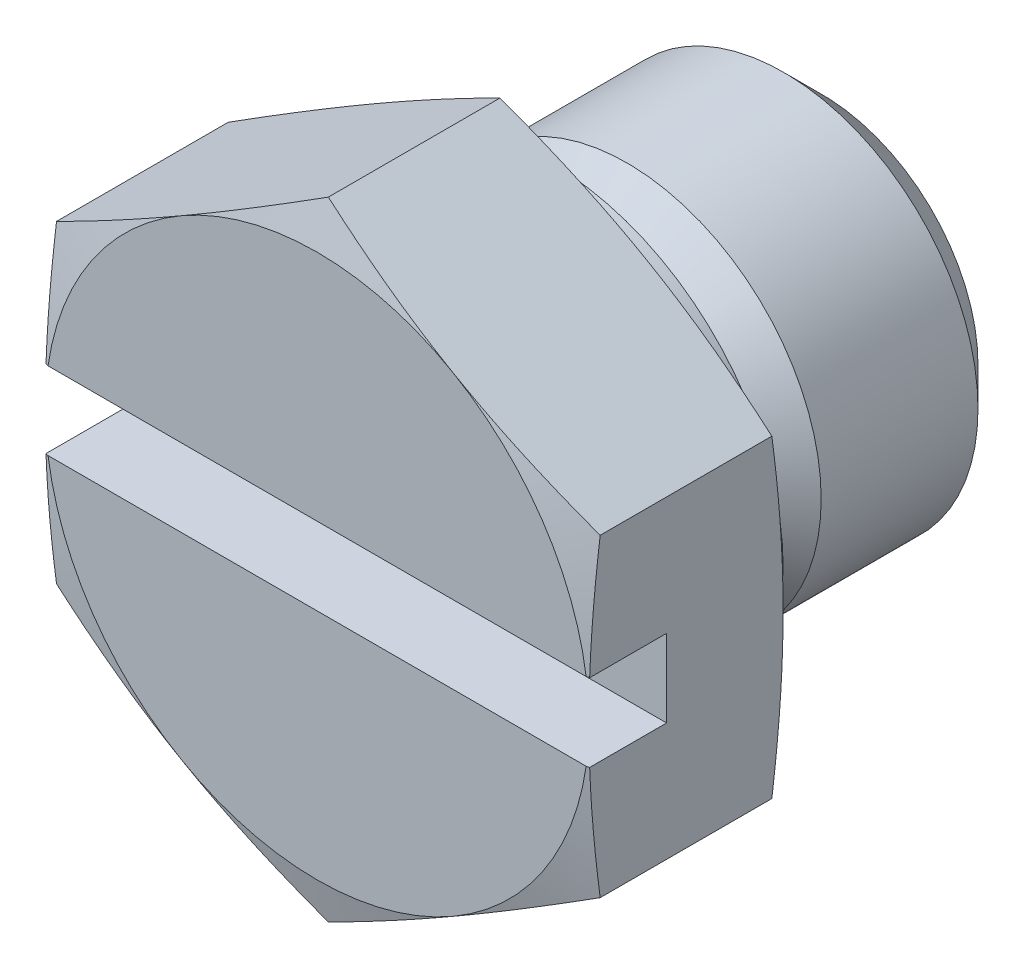
from build123d import *

# Parameters (mm, degrees)
SKETCH_2_R          = 5
CUT_EXTRUDE_1_DEPTH = 3
SKETCH_3_W          = 10
SKETCH_3_H          = 1
CUT_EXTRUDE_2_DEPTH = 1


with BuildPart() as part:
    # 草图1 → 旋转1 (revolve)
    with BuildSketch(Plane(origin=(0, 0, 0), x_dir=(0, 0, -1), z_dir=(1, 0, 0)), mode=Mode.PRIVATE) as revolve_1_sk:
        Polygon((-3, 0), (-3, 3.5), (-2.598076211, 5), (-0.901923789, 5), (-0.5, 3.5), (-0.5, 3), (0, 3), (0, 2.2), (0.5, 2.2), (0.5, 2.0095), (0.9905, 2.5), (3.0095, 2.5), (3.5, 2.0095), (3.5, 0), align=None)
    revolve(revolve_1_sk.sketch.rotate(Axis((0, 0, -3.5), (0, 0, 1)), 270), axis=Axis((0, 0, -3.5), (0, 0, 1)))

    # 草图2 → 切除-拉伸1 (cut)
    with BuildSketch(Plane.XY):
        Circle(SKETCH_2_R)
        Polygon((-3.5, 2.020725942), (-3.5, -2.020725942), (0, -4.041451884), (3.5, -2.020725942), (3.5, 2.020725942), (0, 4.041451884), align=None, mode=Mode.SUBTRACT)
    extrude(amount=CUT_EXTRUDE_1_DEPTH, mode=Mode.SUBTRACT)

    # 草图3 → 切除-拉伸2 (cut)
    with BuildSketch(Plane.XY.offset(3)):
        Rectangle(SKETCH_3_W, SKETCH_3_H)
    extrude(amount=-CUT_EXTRUDE_2_DEPTH, mode=Mode.SUBTRACT)


solid = part.part
